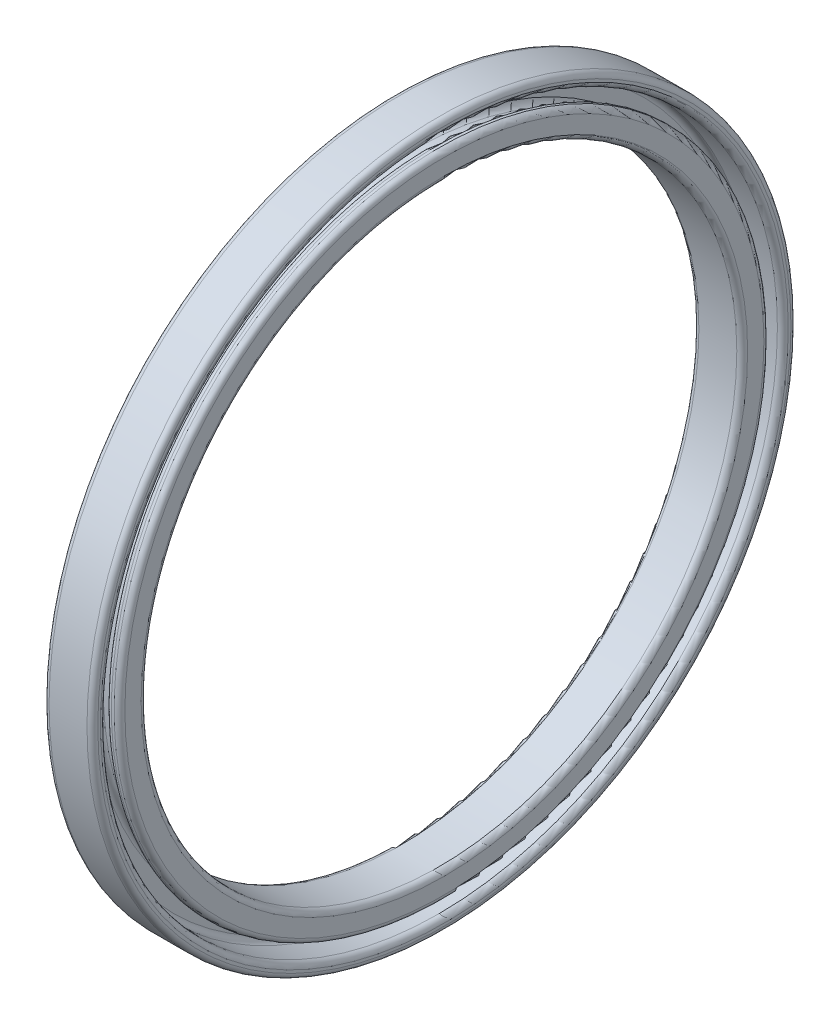
from build123d import *


with BuildPart() as part:
    # Sketch1 → Revolve1 (revolve)
    with BuildSketch(Plane.XY, mode=Mode.PRIVATE) as revolve1_sk:
        with BuildLine():
            Line((2, 110), (16, 110))
            ThreePointArc((16, 110), (17.414213562, 110.585786438), (18, 112))
            Line((18, 112), (18, 118))
            ThreePointArc((18, 118), (17.414213562, 119.414213562), (16, 120))
            Line((16, 120), (15, 120))
            ThreePointArc((15, 120), (13.585786438, 119.414213562), (13, 118))
            Line((13, 118), (13, 117))
            ThreePointArc((13, 117), (12.414213562, 115.585786438), (11, 115))
            Line((11, 115), (7, 115))
            ThreePointArc((7, 115), (5.585786438, 115.585786438), (5, 117))
            Line((5, 117), (5, 123))
            ThreePointArc((5, 123), (5.585786438, 124.414213562), (7, 125))
            Line((7, 125), (16, 125))
            ThreePointArc((16, 125), (17.414213562, 125.585786438), (18, 127))
            Line((18, 127), (18, 128))
            ThreePointArc((18, 128), (17.414213562, 129.414213562), (16, 130))
            Line((16, 130), (2, 130))
            ThreePointArc((2, 130), (0.585786438, 129.414213562), (0, 128))
            Line((0, 128), (0, 112))
            ThreePointArc((0, 112), (0.585786438, 110.585786438), (2, 110))
        make_face()
    revolve(revolve1_sk.sketch.rotate(Axis((119.308058872, 0, 0), (-1, 0, 0)), 90), axis=Axis((119.308058872, 0, 0), (-1, 0, 0)))


solid = part.part
